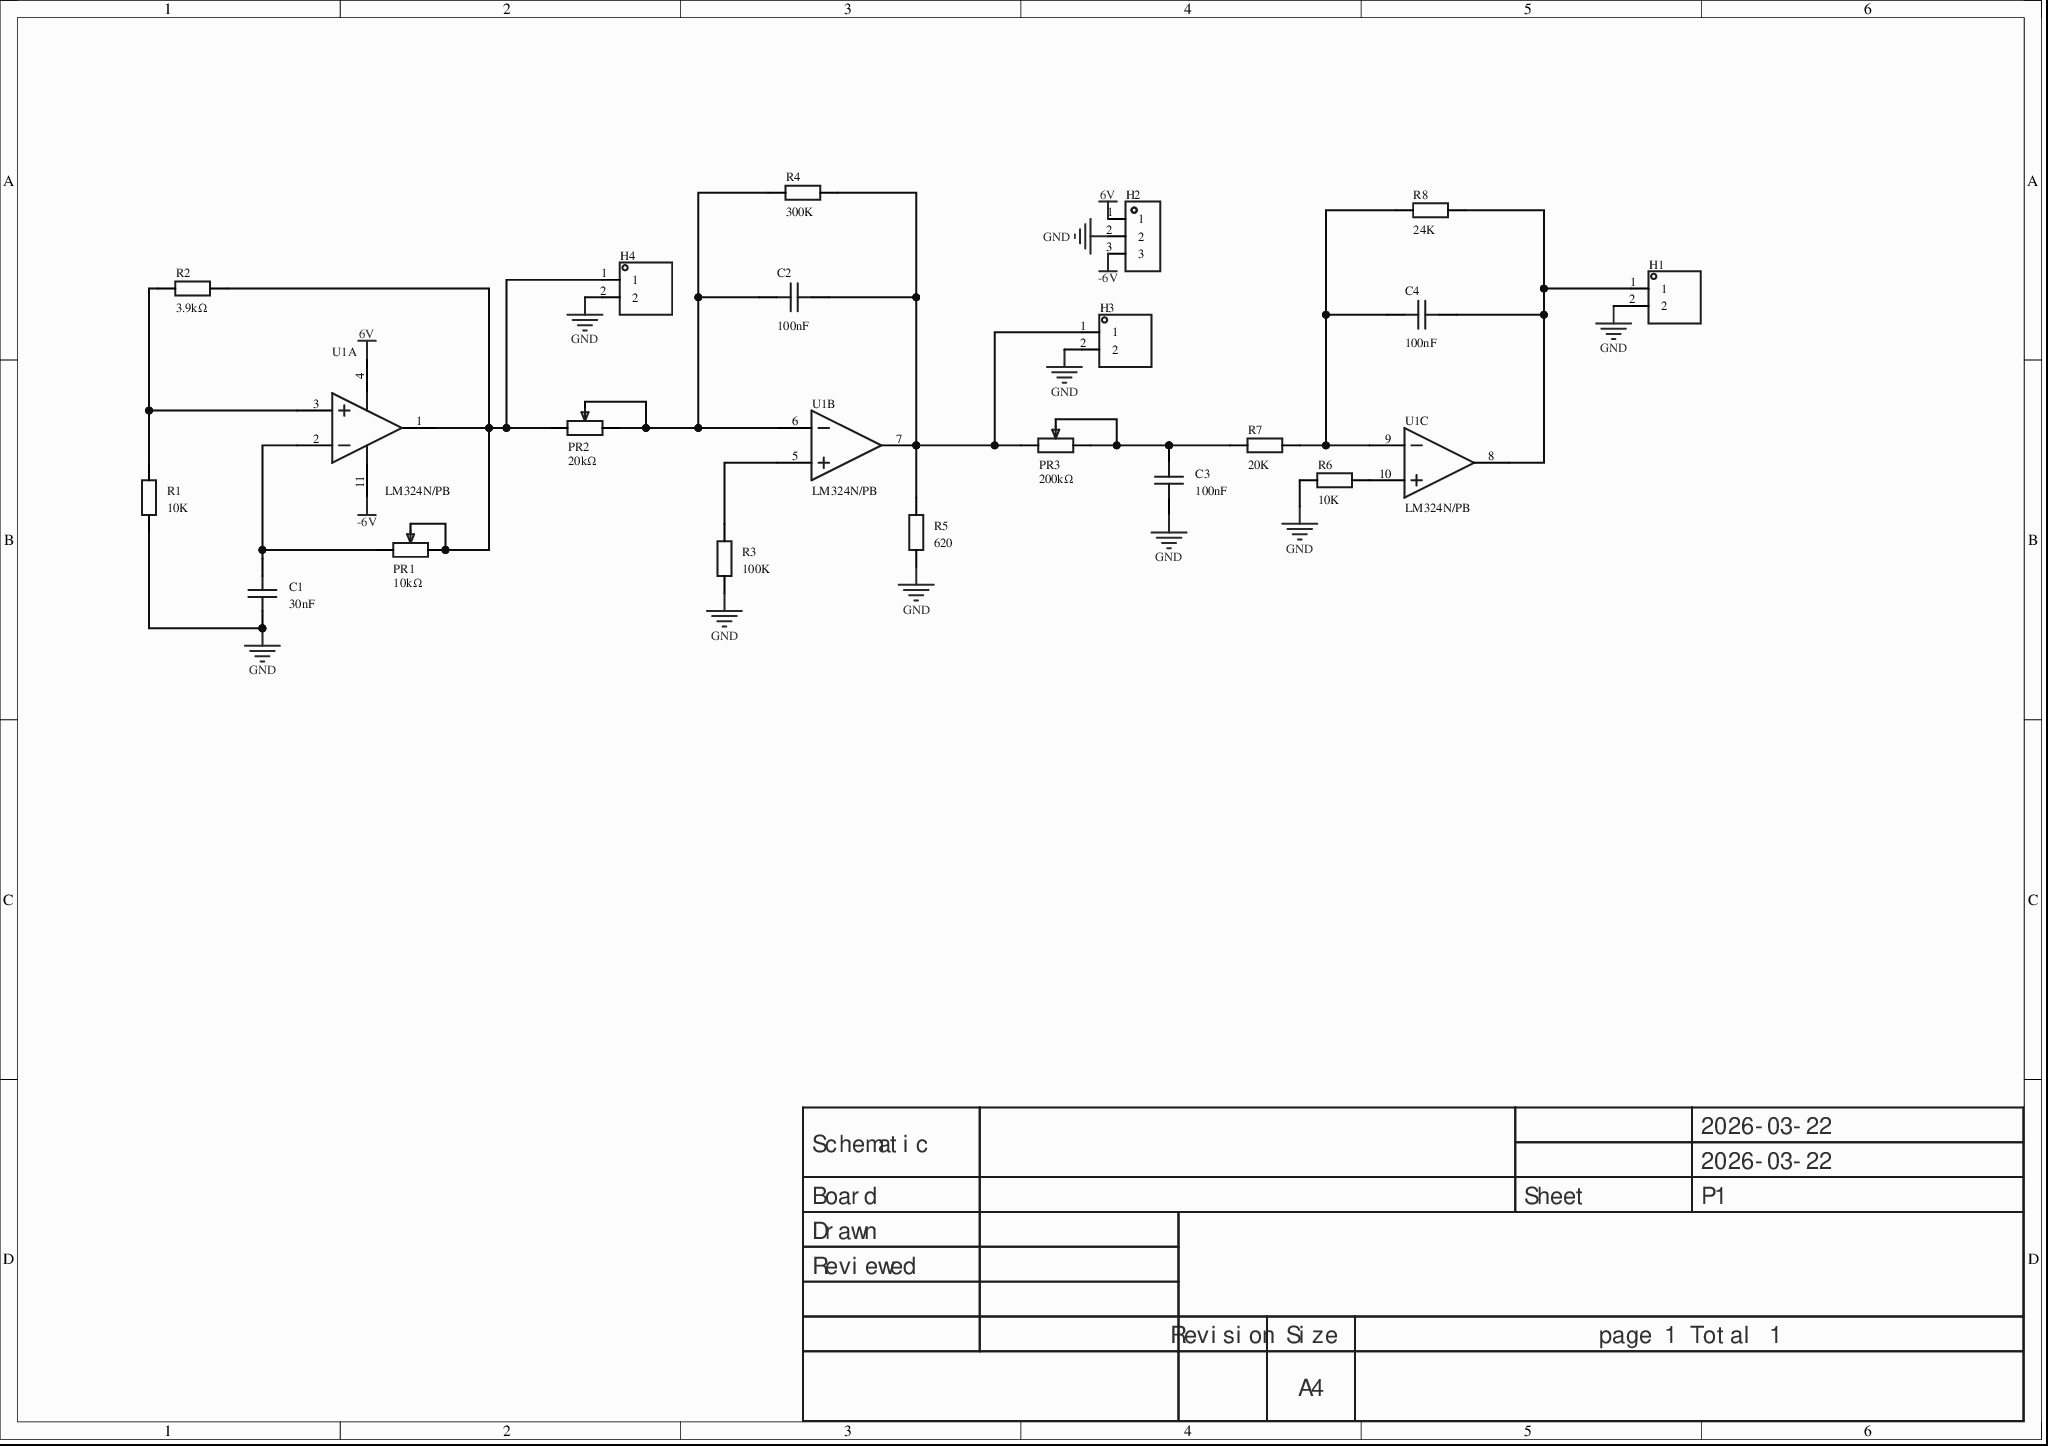
[diagram p0: MISC52110-3.schdoc]
# Altium project MISC52110-2.PrjPcb
1 sheet, 20 parts. Net scope: global (net labels, ports and power ports of the same name join across sheets).
Board file: MISC52110.pcbdoc

## Sheet MISC52110-3.schdoc
size 297 x 209 mm; Version: V1.0; @Project Name: MISC52110; @Update Date: 2026-03-22; @Create Date: 2026-03-22; @Board Name: MISC52110; @Create Time: 13:45:22; @Page Count: 1; @Page No: 1; @Schematic Name: MISC52110; @Update Time: 13:45:22; Size: A4

### Parts
C1  30nF  [C0603]
C2  100nF  [C0603]
C3  100nF  [C0603]
C4  100nF  [C0603]
H1  (no value)  [HDR-TH_2P-P2.54-V-M-1]
H2  (no value)  [HDR-TH_3P-P2.54-V-M]
H3  (no value)  [HDR-TH_2P-P2.54-V-M-1]
H4  (no value)  [HDR-TH_2P-P2.54-V-M-1]
PR1  10kΩ  [R_3296]
PR2  20kΩ  [R_3296]
PR3  200kΩ  [R_3296]
R1  10K  [R0603]
R2  3.9kΩ  [R0603]
R3  100K  [R0603]
R4  300K  [R0603]
R5  620  [R0603]
R6  10K  [R0603]
R7  20K  [R0603]
R8  24K  [R0603]
U1  LM324N/PB  [PDIP-14_L19.2-W6.6-P2.54-LS7.6-BL]  (parts A,B,C of 4)

### Nets
6V: H2.1 U1.4(V+)
-6V: H2.3 U1.11(GND)
GND: C1.1 C3.1 H1.2 H2.2 H3.2 H4.2 R1.1 R3.1 R5.1 R6.1
NetC1_2: C1.2 PR1.3 U1.2(INA+)
NetC2_1: C2.1 PR2.1 PR2.2 R4.1 U1.6(INB-)
NetC2_2: C2.2 H3.1 PR3.3 R4.2 R5.2 U1.7(OUTB)
NetC3_2: C3.2 PR3.1 PR3.2 R7.1
NetC4_1: C4.1 R7.2 R8.1 U1.9(INC-)
NetC4_2: C4.2 H1.1 R8.2 U1.8(OUTC)
NetH4_1: H4.1 PR1.1 PR1.2 PR2.3 R2.1 U1.1(OUTA)
NetR1_2: R1.2 R2.2 U1.3(INA-)
NetR3_2: R3.2 U1.5(INB+)
NetR6_2: R6.2 U1.10(INC+)

### Notes on the sheet
- 2026-03-22
- Schematic
- Board
- Sheet
- P1
- Drawn
- Reviewed
- Revision
- Size
- A4
- page 1 Total 1

### Library data of the parts
C1-C4 = CAP_0603: Symbol: Capacitance; ConvertToPcb: yes; ModelId: ac125912035d415993ca9572d50418b10819f05c4eef4c71ace90d822a990e87; ModelName: C0603_L1.6-W0.8-H0.8; ModelTransform: 62.992,31.496,0,0,0,0,0,0,0; Device: CAP_0603; AddInBom: yes; Supplier Footprint: 0603; FootprintName: C0603
  C1: Value: 30nF
  C2-C4: Value: 100nF
H1 H3 H4 = HDR-M_2.54_1x2P: Symbol: 210S-1*2P L=11.6MMGold-plated black; ConvertToPcb: yes; ModelId: 79b2e9f2d70a4d68a1b7098f27c6d4c50819f05c4eef4c71ace90d822a990e87; ModelName: HDR-M-2.54_1x2; ModelTransform: 200,100,0,0,0,0,0,0,-118.11; Device: HDR-M_2.54_1x2P; AddInBom: yes; SupplierPart: C124375; Supplier Footprint: 插件; FootprintName: HDR-TH_2P-P2.54-V-M-1
H2 = HDR-M_2.54_1x3P: AddInBom: yes; ModelId: bb473b6d38ff42a99216a4fcdbdcc4cb0819f05c4eef4c71ace90d822a990e87; ModelName: HDR-TH_3P-P2.54-M-LI-1X3P; ModelTransform: 300.03877,100,0,0,0,0,0,0,-118.11; Symbol: HDR-M_2.54_1x3P; Device: HDR-M_2.54_1x3P; ConvertToPcb: yes; FootprintName: HDR-TH_3P-P2.54-V-M; SupplierPart: C2937625; Supplier Footprint: 插件
PR1-PR3 = R_3296: ConvertToPcb: yes; ModelId: b182808559bb43bda9e7de64b64134cb0819f05c4eef4c71ace90d822a990e87; ModelName: 3296W; ModelTransform: 373.98,188.96,590.49,180,0,0,0,0,-140; Symbol: R_3296; Device: R_3296; AddInBom: yes; Supplier Footprint: 直插; FootprintName: R_3296
  PR1: Value: 10kΩ
  PR2: Value: 20kΩ
  PR3: Value: 200kΩ
R1-R8 = Res_0603: Symbol: Resistor; ConvertToPcb: yes; ModelId: fc143cca1e79419f9cd78b61e9279f080819f05c4eef4c71ace90d822a990e87; ModelTransform: 31.8897,63.7794,0,90,0,0,0,0,0; Device: Res_0603; AddInBom: yes; Supplier Footprint: 0603; FootprintName: R0603; ModelName: R0603
  R1 R6: Value: 10K
  R2: Value: 3.9kΩ
  R3: Value: 100K
  R4: Value: 300K
  R5: Value: 620
  R7: Value: 20K
  R8: Value: 24K
U1 = LM324N/PB: LM324N/PB component. Amplifiers: quad; gain-bandwidth product (GBP): 1MHz; input bias current (Ib): 45nA;; Manufacturer: TI(德州仪器); Relevance: []; AddInBom: yes; ModelId: 08aeb3774ab0450ba412f07c9830bd710819f05c4eef4c71ace90d822a990e87; ModelTransform: 755.904,309.842,0,0,0,0,0,0,-129.921; Output Current: 40mA; Symbol: LM324N/PB; Device: LM324N/PB; LCSC Part Name: LM324N/PB; SupplierPart: C4366406; ManufacturerPart: LM324N/PB; Supplier Footprint: PDIP-14; JLCPCB Part Class: Extended Part; Datasheet: https://atta.szlcsc.com/upload/public/pdf/source/20230921/264342EF71D0FEA3F079F4D0F511985F.pdf; Supplier: LCSC; ConvertToPcb: yes; FootprintName: PDIP-14_L19.2-W6.6-P2.54-LS7.6-BL; ModelName: PDIP-14_L19.2-W6.6-P2.54-LS7.6-BL; Number of Circuits: Quad; Gain Bandwidth Product(GBP): 1MHz; Current - Input Bias(Ib): 45nA; Operating Temperature: 0℃~+70℃